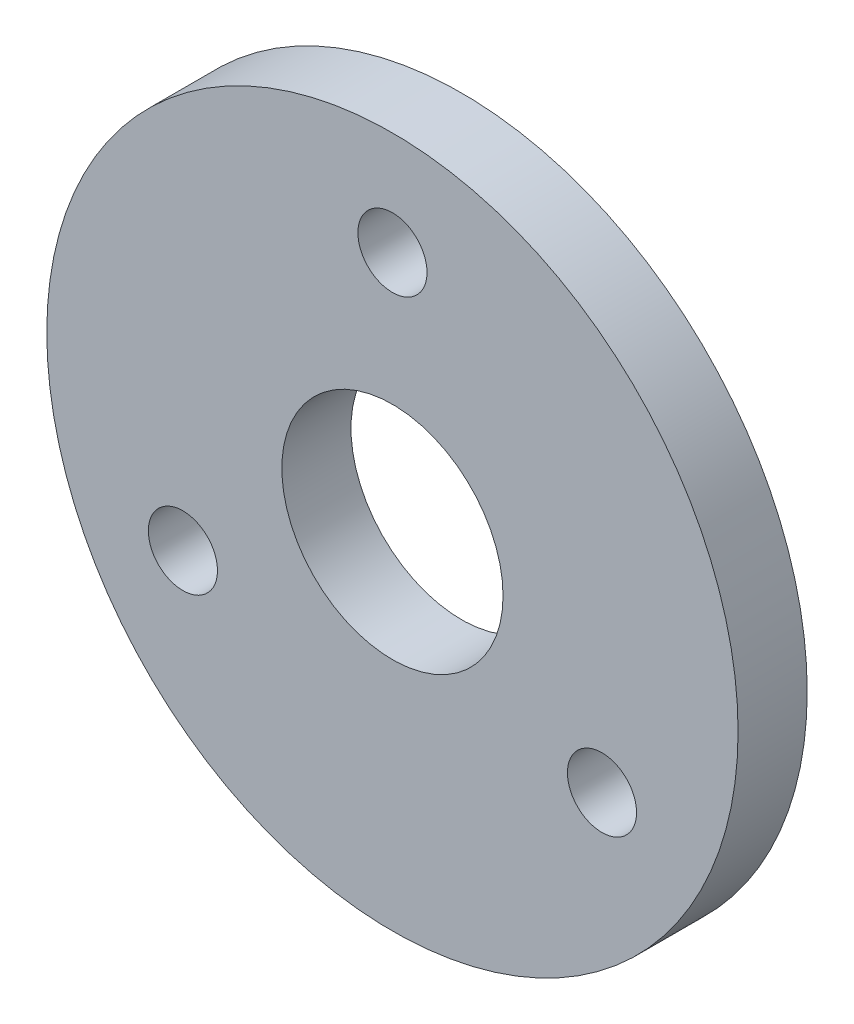
from build123d import *

# Parameters (mm, degrees)
SKETCH1_R           = 50
BOSS_EXTRUDE1_DEPTH = 10
SKETCH2_R           = 5
CUT_EXTRUDE1_DEPTH  = 10
CIRPATTERN1_COUNT   = 3
SKETCH3_R           = 16
CUT_EXTRUDE2_DEPTH  = 10


with BuildPart() as part:
    # Sketch1 → Boss-Extrude1 (new body)
    with BuildSketch(Plane.XY):
        Circle(SKETCH1_R)
    extrude(amount=BOSS_EXTRUDE1_DEPTH)

    # Sketch2 → Cut-Extrude1 (cut)
    with BuildSketch(Plane.XY.offset(10)):
        with Locations((0, 35)):
            Circle(SKETCH2_R)
    cut_extrude1 = extrude(amount=-CUT_EXTRUDE1_DEPTH, mode=Mode.SUBTRACT)

    # CirPattern1: Cut-Extrude1 ×3 about axis
    cirpattern1_axis = Axis((0, 0, 0), (0, 0, 1))
    for i in range(1, CIRPATTERN1_COUNT):
        add(cut_extrude1.rotate(cirpattern1_axis, i * 360 / CIRPATTERN1_COUNT), mode=Mode.SUBTRACT)

    # Sketch3 → Cut-Extrude2 (cut)
    with BuildSketch(Plane.XY.offset(10)):
        Circle(SKETCH3_R)
    extrude(amount=-CUT_EXTRUDE2_DEPTH, mode=Mode.SUBTRACT)


solid = part.part
